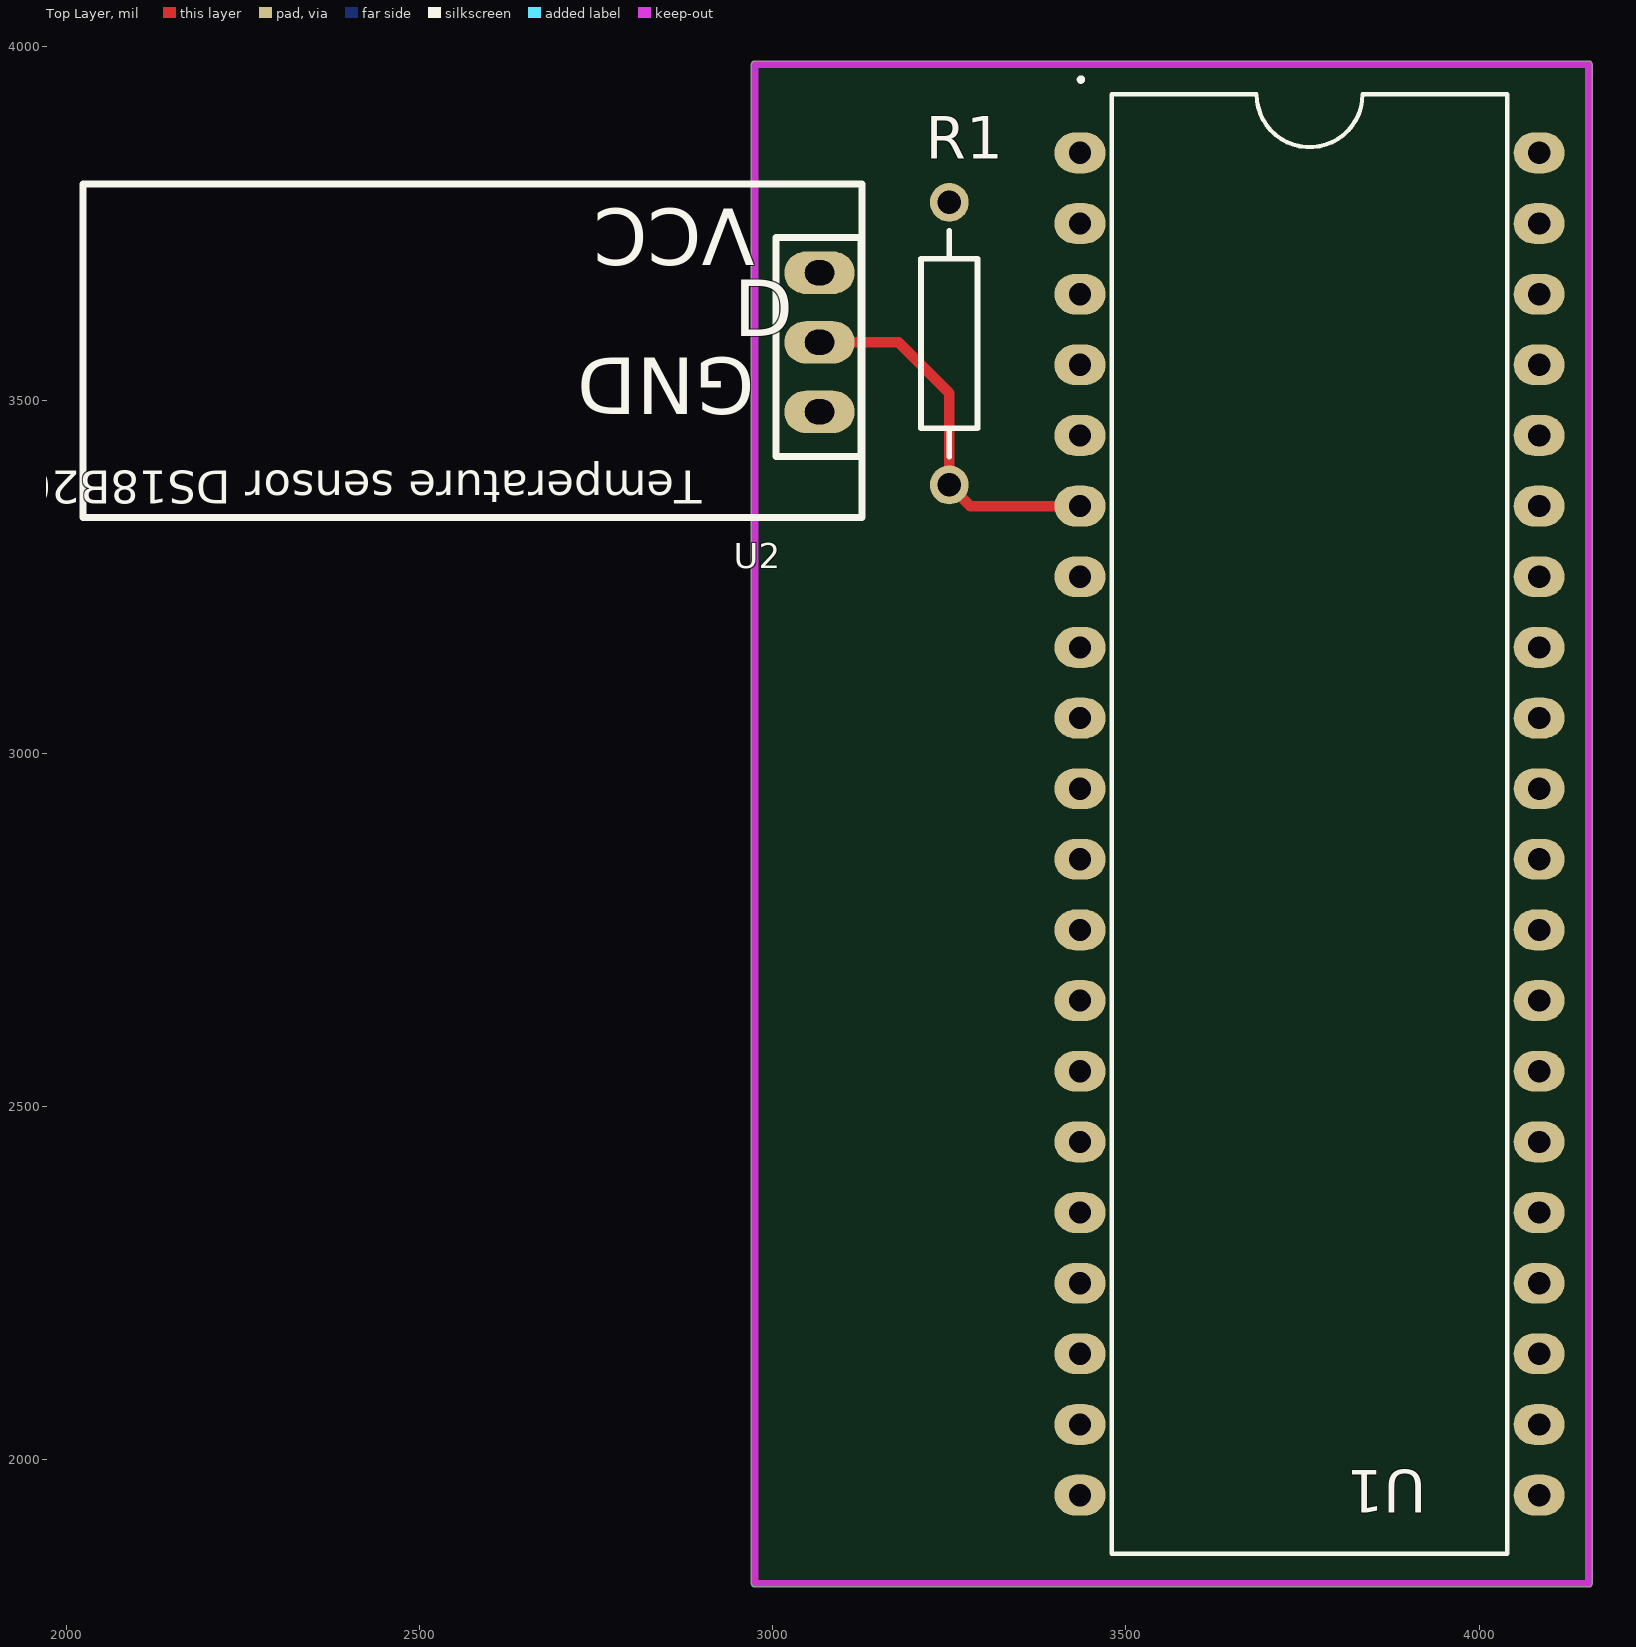
[diagram p0: Top Layer view]
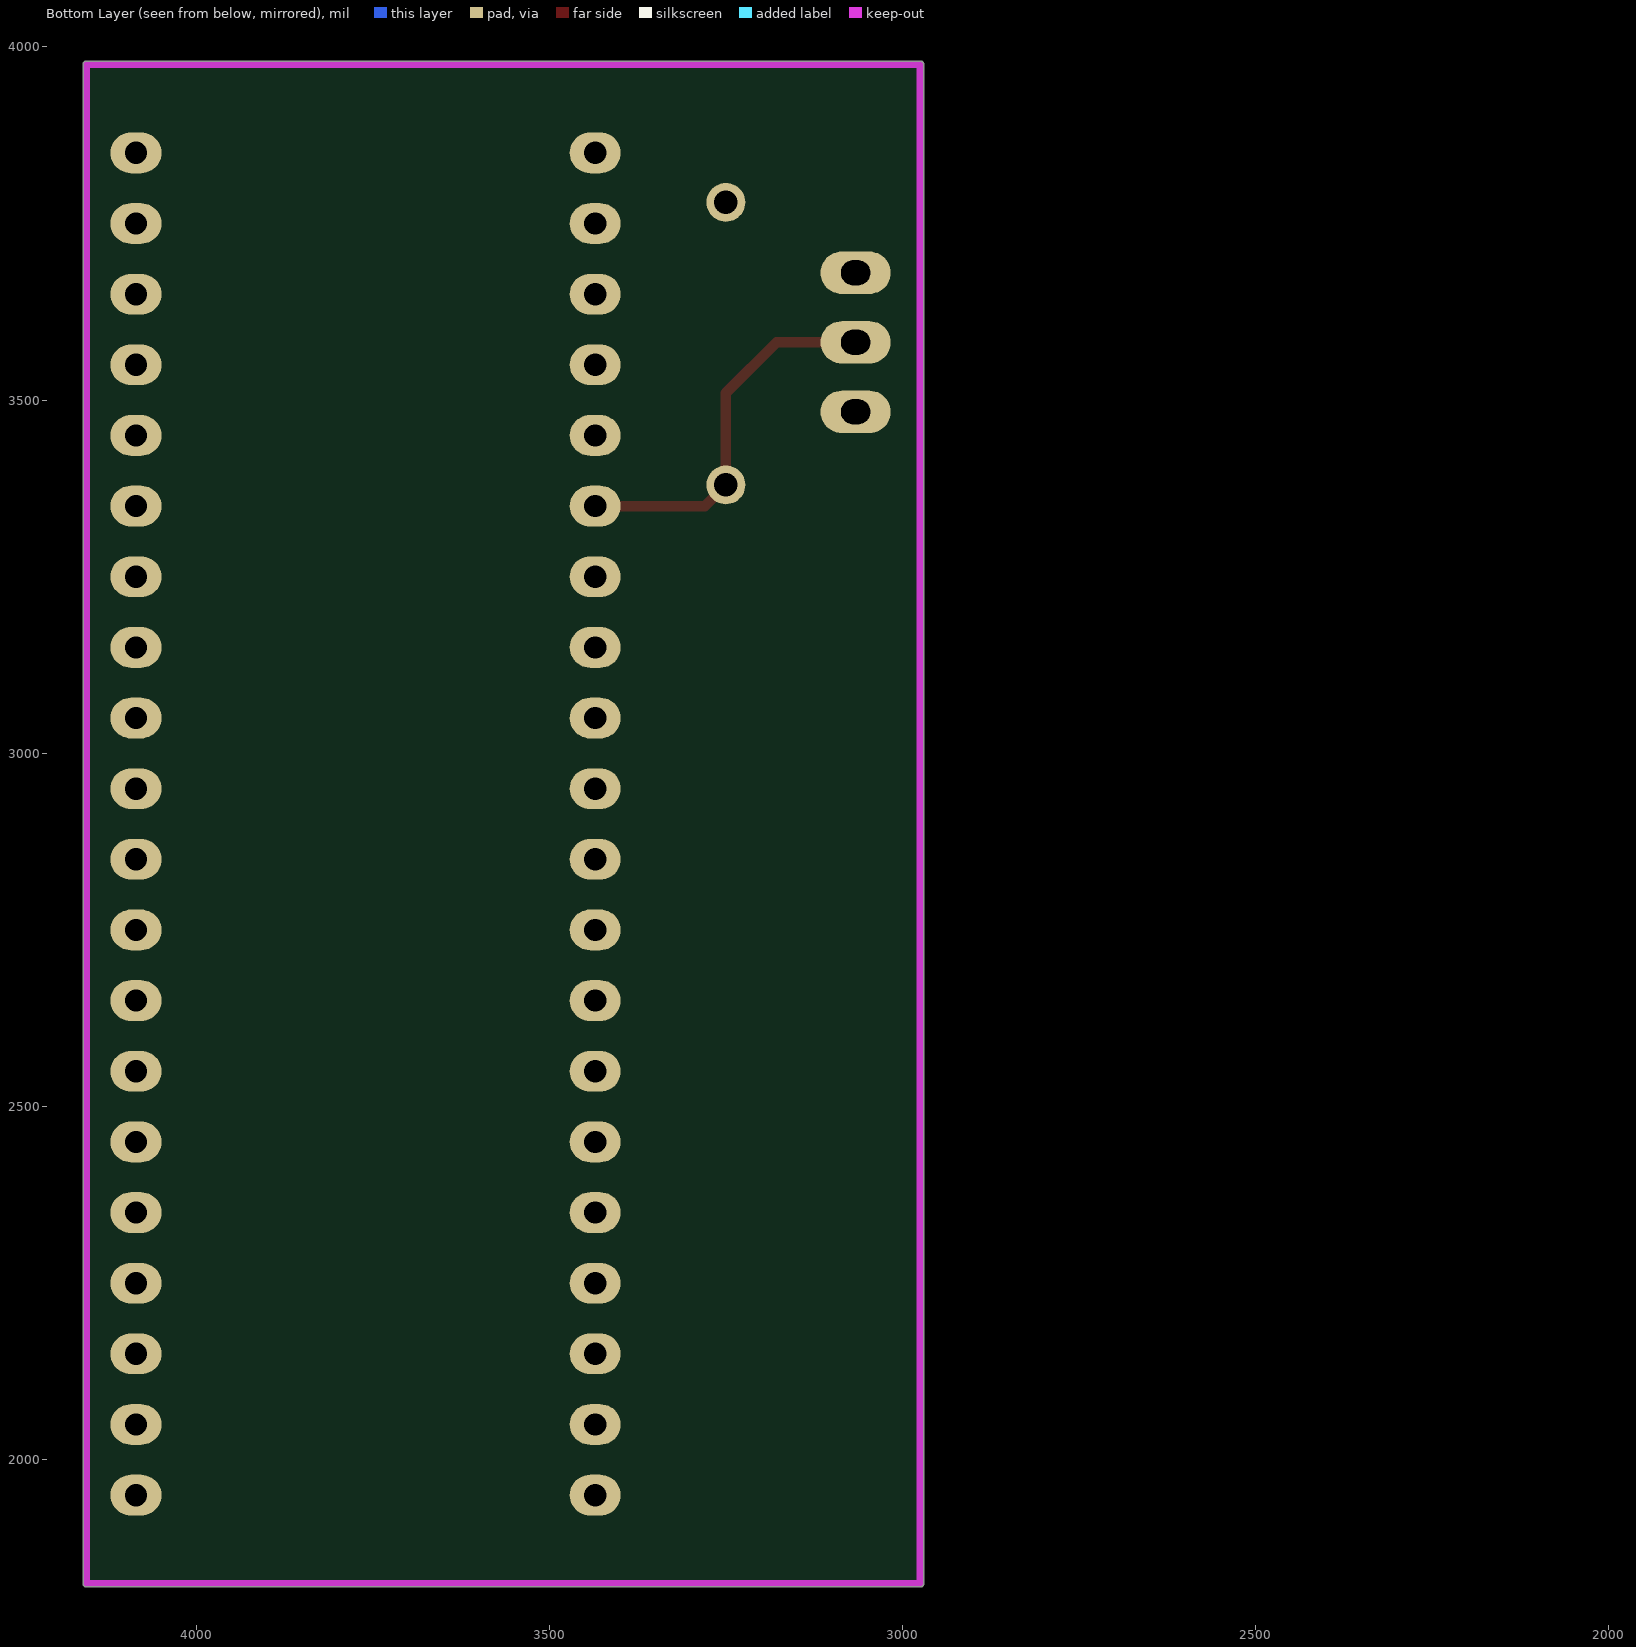
[diagram p1: Bottom Layer view, seen from below]
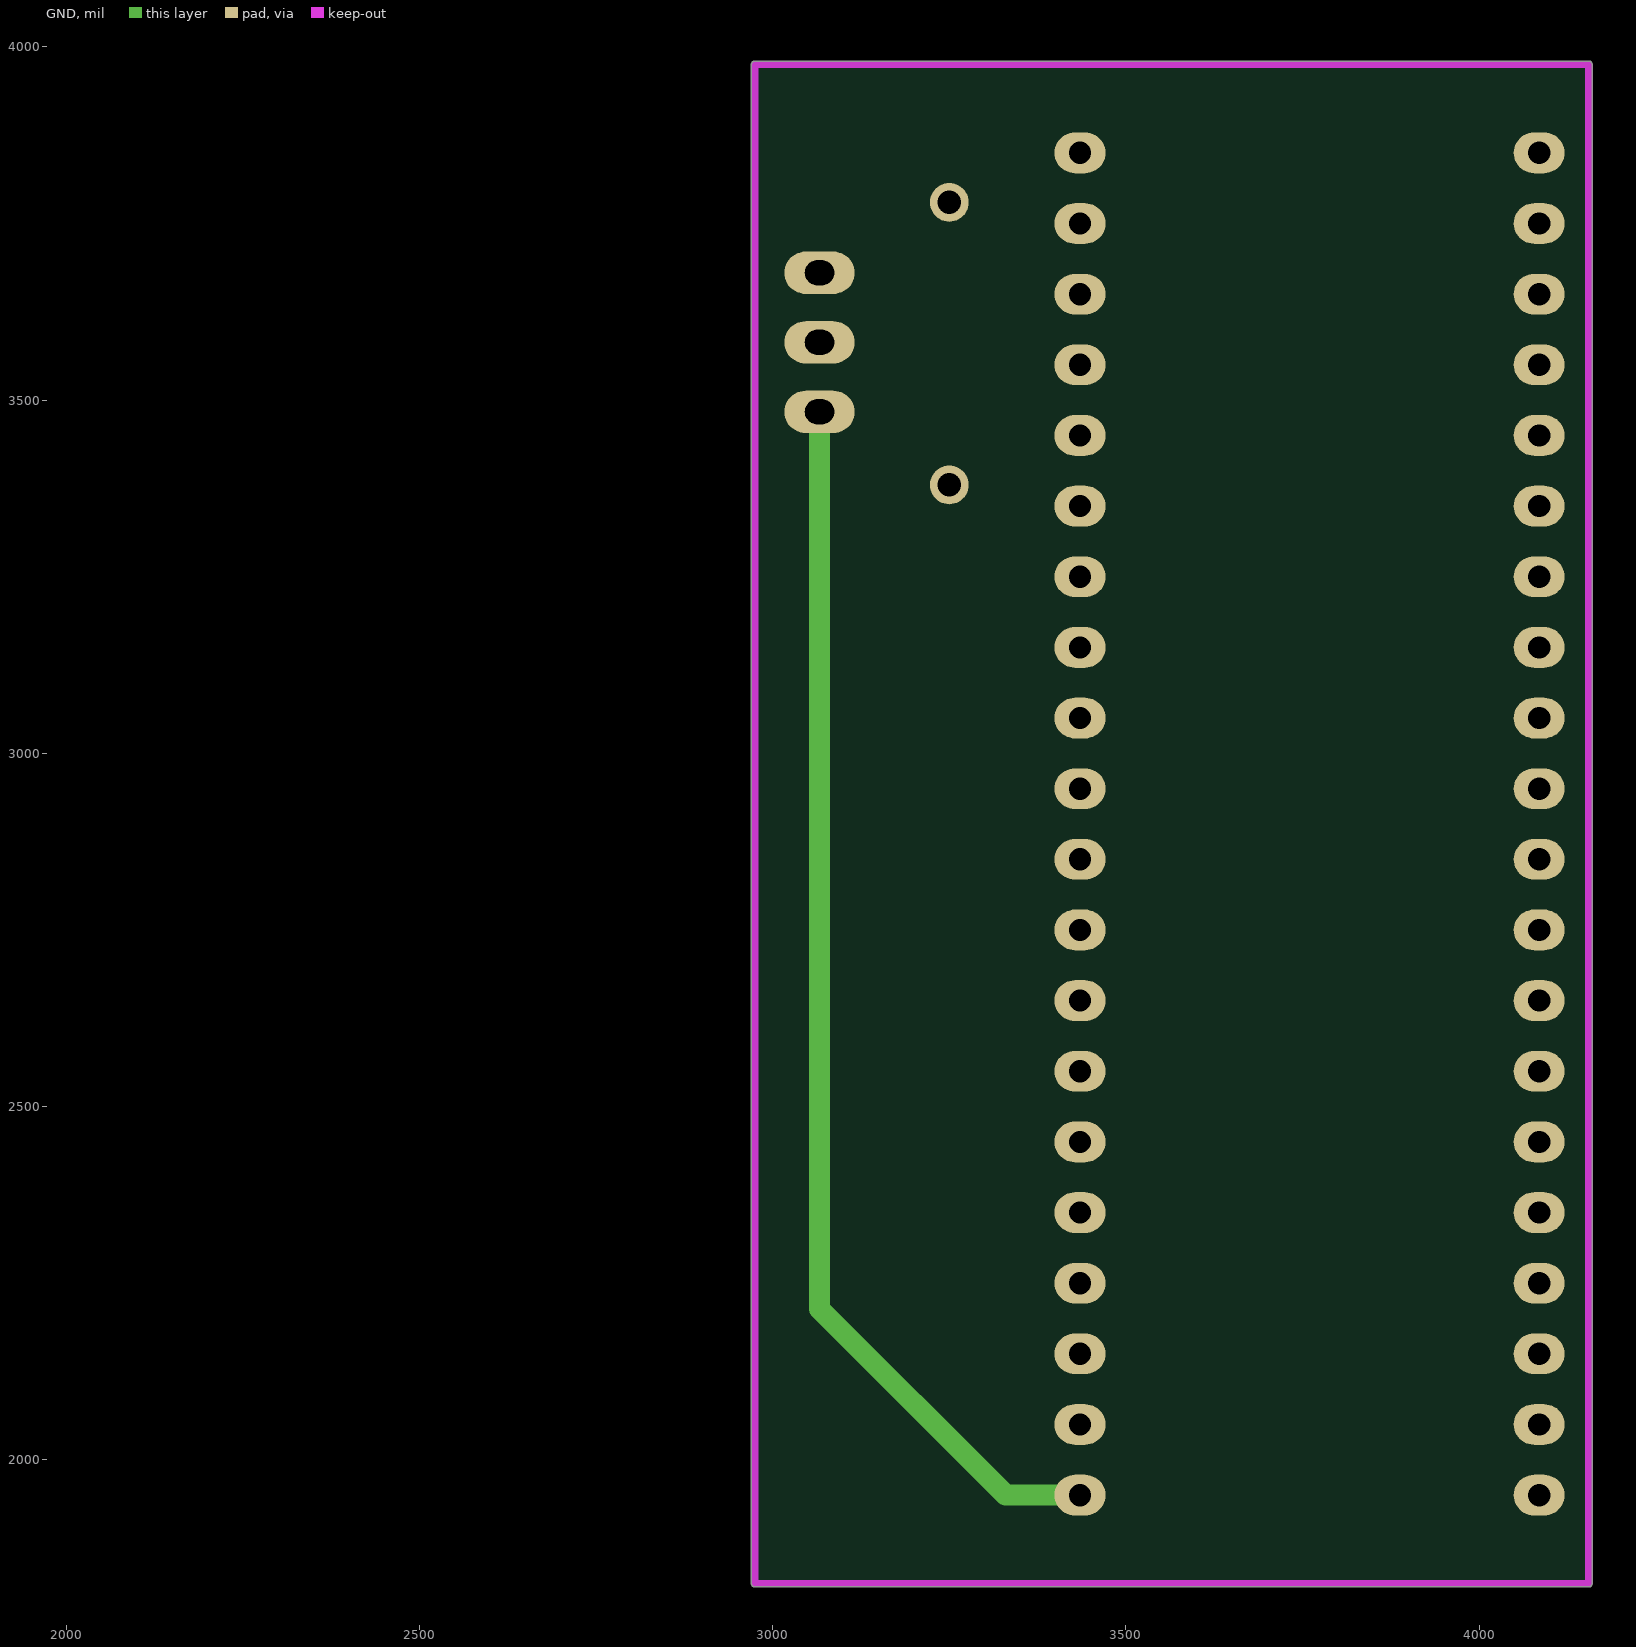
[diagram p2: GND]
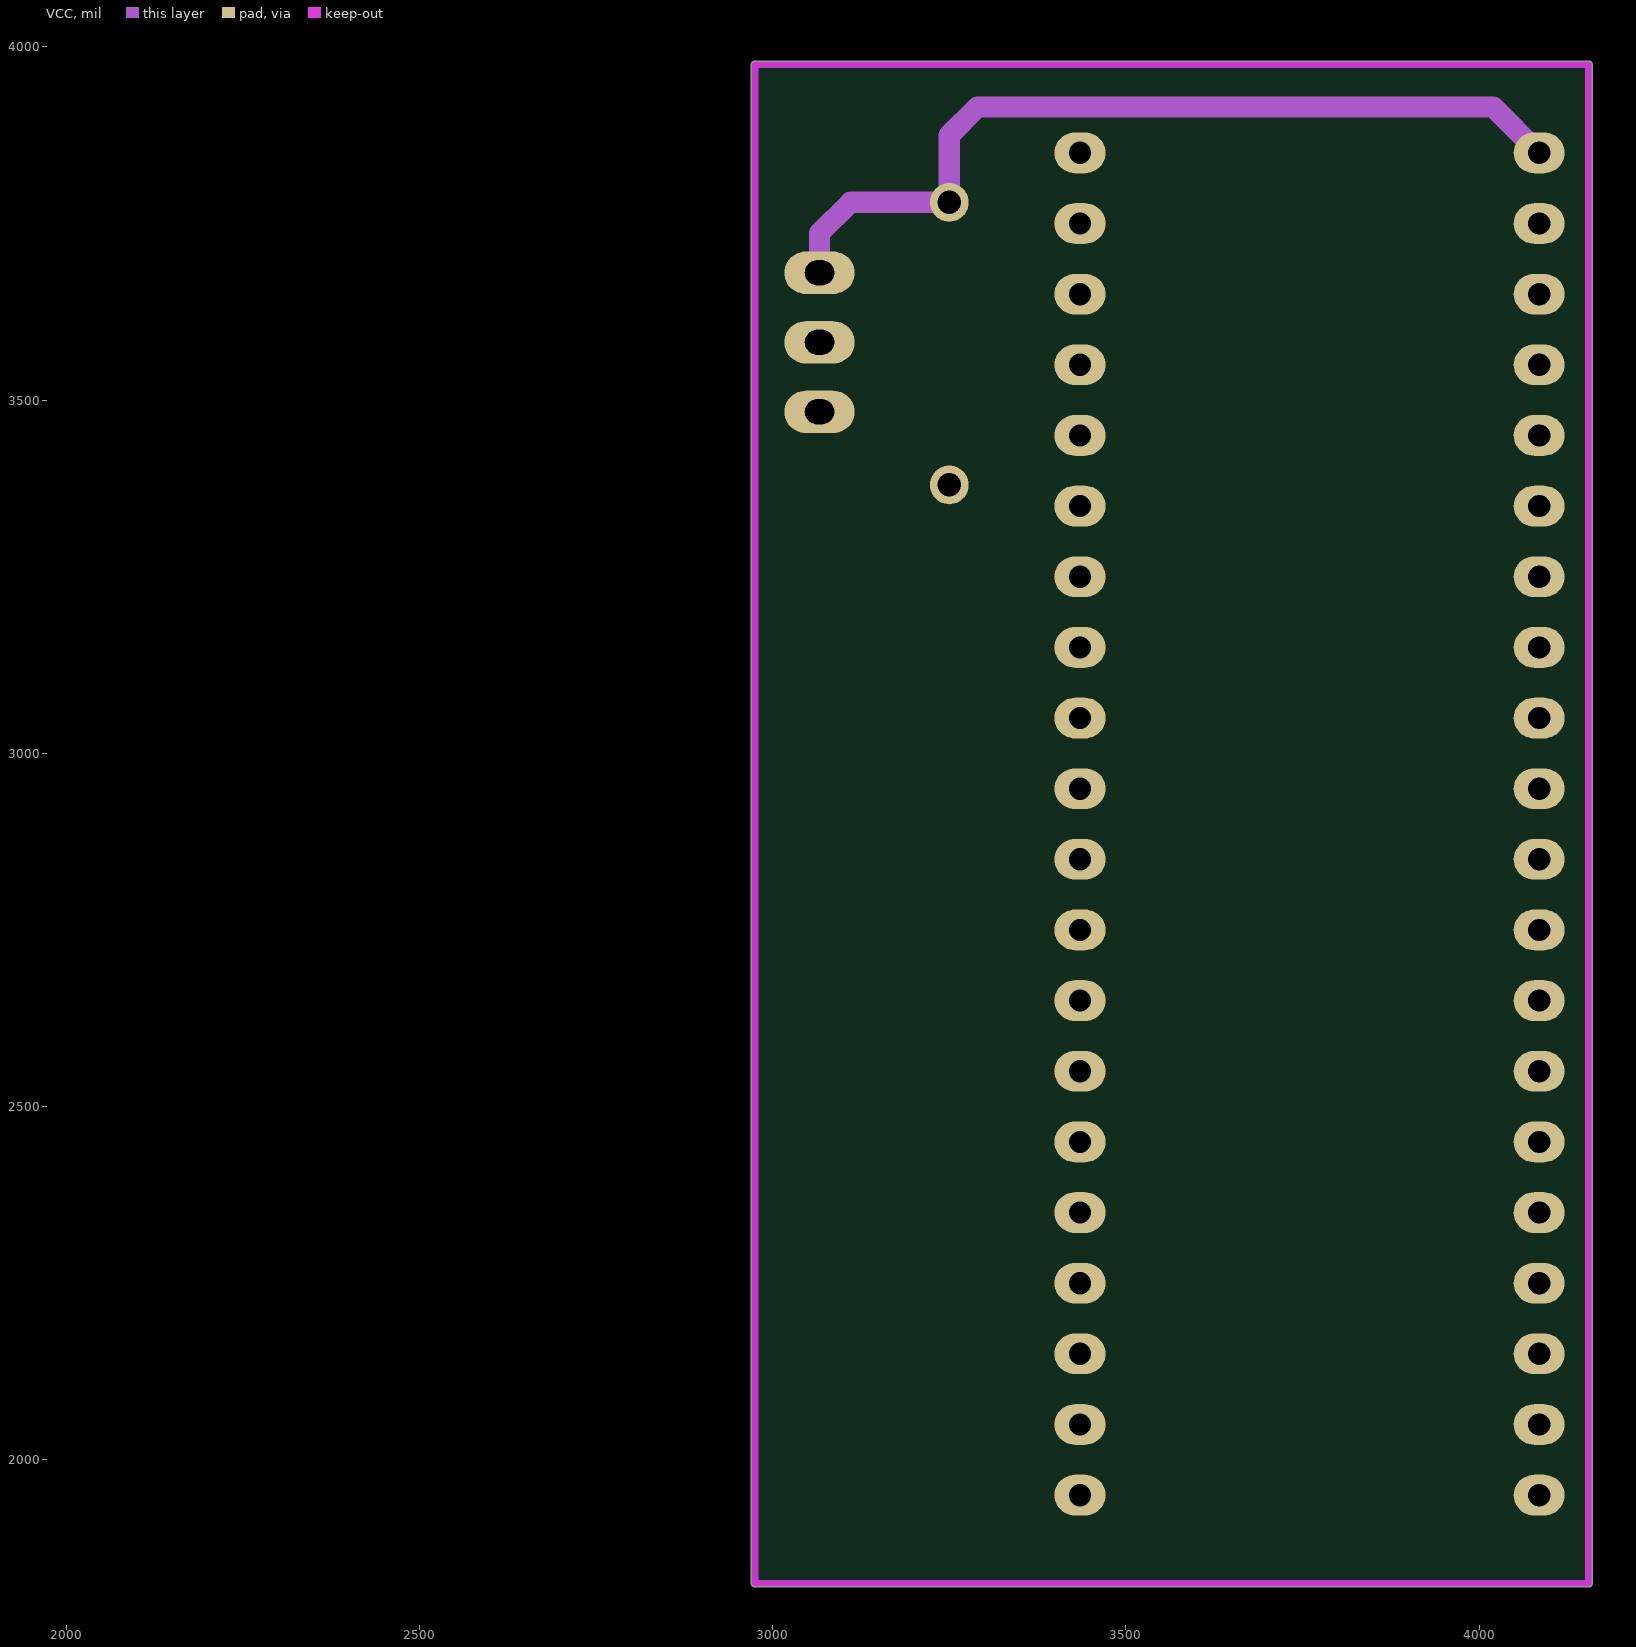
[diagram p3: VCC]
# Altium PCB MISC82899.PcbDoc
Units mil, origin at the board's own origin, x right, y up, seen from the top; angles counter-clockwise.
Board outline 1190.03 x 2160.03 mil, 4 copper layers (Top Layer, GND, VCC, Bottom Layer), stack 30.634 mil thick; 3 components, 3 nets, 45 pads, 0 vias.

## Layer stack, top to bottom
Top Solder: solder mask 0.4, Solder Resist, Dk 3.5
Top Layer: signal copper 1.4
Dielectric 1: core 10, FR-4, Dk 4.2
GND: signal copper 1.417
Dielectric 4: prepreg 5, Dk 4.2
VCC: signal copper 1.417
Dielectric 3: core 10, Dk 4.2
Bottom Layer: signal copper 1.4
Bottom Solder: solder mask 0.4, Solder Resist, Dk 3.5

## Board outline
2969.99,1825 ccw(c2975,1825) 2975,1819.98 4155,1819.98 ccw(c4155,1825) 4160.02,1825 4160.02,3975 ccw(c4155,3975) 4155,3980.01 2975,3980.01 ccw(c2975,3975) 2969.99,3975

## Design rules (kind name [scope] priority, off if disabled: settings)
Clearance [All] p1: gap=10
MinimumSolderMaskSliver [All] p1: minsoldermaskwidth=0
PolygonConnect [All] p1: connectstyle=Relief reliefconductorwidth=10 reliefentries=4 polygonreliefangle="90 Angle" airgapwidth=10
RoutingVias [All] p1: holewidth=28 width=50 viastyle="Through Hole" minholewidth=28 minwidth=50 maxholewidth=28 maxwidth=50
SilkToSilkClearance [All] p1: silktosilkclearance=0
SilkToSolderMaskClearance [IsPad] p1: minsilkscreentomaskgap=0 clearancetoexposedcopper=TRUE
SolderMaskExpansion [All] p1: expansion=4
Width [All] p1: maxlimit=30 minlimit=10 preferedwidth=10
27 further rules are at their usual default settings.

## Components (designator, comment, footprint, x,y, rotation, side; value= is the part's Value field where it differs from the comment)
R1 "10K" AXIAL-0.4 3250,3580 r90 top
U1 "STC89C52RC" STC89C52RC 3760,2910.33 r270 top
U2 "Comment" DS18B20 2575,3570 r180 top

## Footprints (in the part's own frame and the unit in brackets; to place one, negate y for a bottom-side part, rotate by r counter-clockwise, add the part's x,y. Pads: shape width x height; smd on the part's side, far side on the other; paste and mask are expansions set on the pad)
AXIAL-0.4 [mm] "Axial Device, Thru-Hole; 2 Leads; 0.4 in Pin Spacing"
  round 1.4 hole 0.85: 1(-5.08,0) 2(5.08,0)
  silkscreen extent -4.06,-1.02 4.06,1.02
DS18B20 [mil]
  oval 99.37x60 hole 35.43 slot 41.34 at 0 deg paste+0 mask+4: 1(-491.35,86.55) 2(-491.35,-11.88) 3(-491.35,-110.3)
  silkscreen extent -551,-236 551,236
STC89C52RC [mm]
  oval 1.467x1.833 hole 0.8 paste+0 mask+0.051: 1(-23.868,-8.255) 2(-21.328,-8.255) 3(-18.788,-8.255) 4(-16.248,-8.255) 5(-13.708,-8.255) 6(-11.168,-8.255) 7(-8.628,-8.255) 8(-6.088,-8.255) 9(-3.548,-8.255) 10(-1.008,-8.255) 11(1.532,-8.255) 12(4.072,-8.255) 13(6.612,-8.255) 14(9.152,-8.255) 15(11.692,-8.255) 16(14.232,-8.255) 17(16.772,-8.255) 18(19.312,-8.255) 19(21.852,-8.255) 20(24.392,-8.255) 21(24.392,8.255) 22(21.852,8.255) 23(19.312,8.255) 24(16.772,8.255) 25(14.232,8.255) 26(11.692,8.255) 27(9.152,8.255) 28(6.612,8.255) 29(4.072,8.255) 30(1.532,8.255) 31(-1.008,8.255) 32(-3.548,8.255) 33(-6.088,8.255) 34(-8.628,8.255) 35(-11.168,8.255) 36(-13.708,8.255) 37(-16.248,8.255) 38(-18.788,8.255) 39(-21.328,8.255) 40(-23.868,8.255)
  silkscreen extent -26.58,-8.3 26.5,7.11

## Part data
R1: library part Res2, "Resistor"

## Nets (pads, with @x,y where several pads share a name; then routed paths per layer and width w, separated by ;. In a path a pad name is that pad's centre, name@x,y a point inside that pad or via, vN(x,y) a via of type N, cw(c..) or ccw(c..) an arc to the next point about the centre after c; other vN are vias at no path point)
GND: U1.20 U2.1 | length 1747.7
  GND w30: U2.1 3066.35,2213.65 3330,1950 U1.20
NetR1_1: R1.1 U1.6 U2.2 | length 540.9
  Top Layer w15: U2.2 3178.12,3581.88 3250,3510 R1.1 3280,3350 U1.6
VCC: R1.2 U1.40 U2.3 | length 1231.3
  VCC w30: U2.3 3066.35,3736.35 3110,3780 R1.2 3250,3875 3290,3915 4020,3915 U1.40
pads on no net: U1.1 U1.2 U1.3 U1.4 U1.5 U1.7 U1.8 U1.9 U1.10 U1.11 U1.12 U1.13 U1.14 U1.15 U1.16 U1.17 U1.18 U1.19 U1.21 U1.22 U1.23 U1.24 U1.25 U1.26 U1.27 U1.28 U1.29 U1.30 U1.31 U1.32 U1.33 U1.34 U1.35 U1.36 U1.37 U1.38 U1.39

## Keep-outs
Keep-Out Layer:
  lines w10: 4055,3975 4155,3975 4155,1825 2975,1825 2975,3975 4075,3975